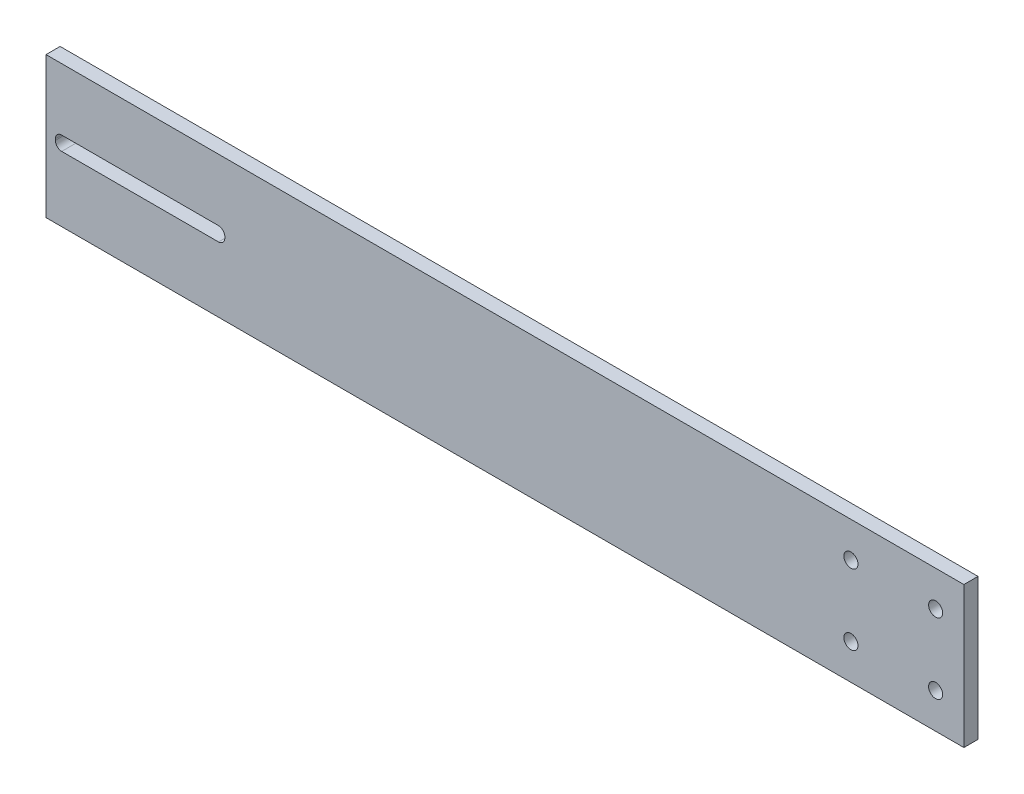
from build123d import *

# Parameters (mm, degrees)
SKETCH1_W           = 650
SKETCH1_H           = 100
BOSS_EXTRUDE1_DEPTH = 10
SKETCH2_R           = 5
CUT_EXTRUDE2_DEPTH  = 10
CUT_EXTRUDE3_DEPTH  = 10


with BuildPart() as part:
    # Sketch1 → Boss-Extrude1 (new body)
    with BuildSketch(Plane.XY):
        Rectangle(SKETCH1_W, SKETCH1_H)
    extrude(amount=BOSS_EXTRUDE1_DEPTH)

    # Sketch2 → Cut-Extrude2 (cut)
    with BuildSketch(Plane.XY.offset(10)):
        with Locations((305, 25)):
            Circle(SKETCH2_R)
        with Locations((245, 25)):
            Circle(SKETCH2_R)
        with Locations((245, -25)):
            Circle(SKETCH2_R)
        with Locations((305, -25)):
            Circle(SKETCH2_R)
    extrude(amount=-CUT_EXTRUDE2_DEPTH, mode=Mode.SUBTRACT)

    # Sketch3 → Cut-Extrude3 (cut)
    with BuildSketch(Plane.XY.offset(10)):
        with BuildLine():
            Line((-313.885022578, -3.814336714), (-202.885022578, -3.814336714))
            ThreePointArc((-202.885022578, -3.814336714), (-199.703042062, -2.496317229), (-198.385022578, 0.685663286))
            Line((-198.385022578, 0.685663286), (-198.385022578, 1.685663286))
            ThreePointArc((-198.385022578, 1.685663286), (-199.703042062, 4.867643802), (-202.885022578, 6.185663286))
            Line((-202.885022578, 6.185663286), (-313.885022578, 6.185663286))
            ThreePointArc((-313.885022578, 6.185663286), (-317.067003093, 4.867643802), (-318.385022578, 1.685663286))
            Line((-318.385022578, 1.685663286), (-318.385022578, 0.685663286))
            ThreePointArc((-318.385022578, 0.685663286), (-317.067003093, -2.496317229), (-313.885022578, -3.814336714))
        make_face()
    extrude(amount=-CUT_EXTRUDE3_DEPTH, mode=Mode.SUBTRACT)


solid = part.part
